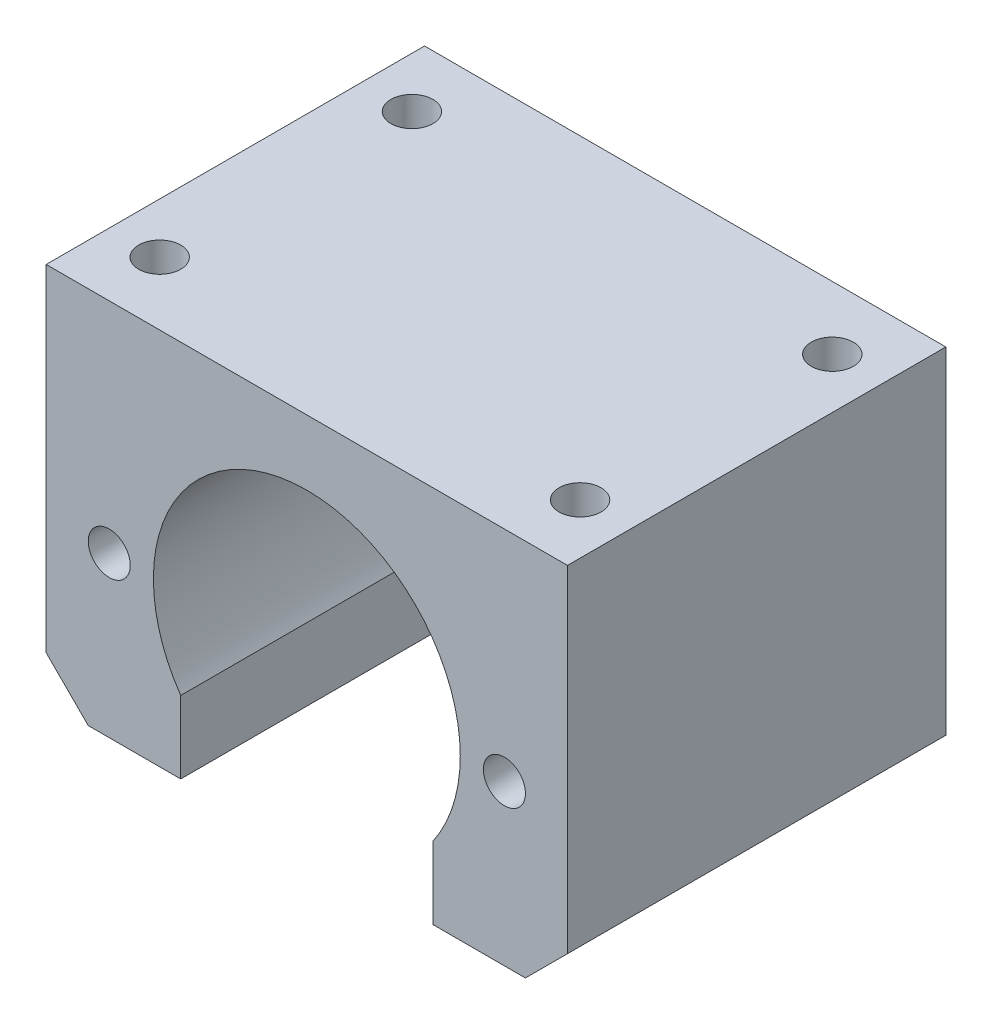
from build123d import *

# Parameters (mm, degrees)
SKETCH_1_W                  = 62
SKETCH_1_H                  = 45
EXTRUDE_1_DEPTH             = 22.5
CUT_EXTRUDE_1_DEPTH         = 45
CHAMFER_1_SIZE              = 5
HOLE_WIZARD_M6_1_D          = 5
HOLE_WIZARD_M6_1_DEPTH      = 15
HOLE_WIZARD_M6_1_TIP        = 1.502151548
HOLE_WIZARD_M6_2_AT_2_COUNT = 2
HOLE_WIZARD_M6_2_AT_2_PITCH = 47


with BuildPart() as part:
    # 草图1 → 凸台-拉伸1 (new, symmetric)
    with BuildSketch(Plane(origin=(0, 0, 0), x_dir=(1, 0, 0), z_dir=(0, 1, 0))):
        Rectangle(SKETCH_1_W, SKETCH_1_H)
    extrude(amount=EXTRUDE_1_DEPTH, both=True)

    # 草图2 → 切除-拉伸1 (cut)
    with BuildSketch(Plane(origin=(0, 0, -22.5), x_dir=(-1, 0, 0), z_dir=(0, 0, -1))):
        with BuildLine():
            Line((-15, -13.895311443), (-15, -22.5))
            Line((-15, -22.5), (15, -22.5))
            Line((15, -22.5), (15, -13.895311443))
            ThreePointArc((15, -13.895311443), (0, 14.75), (-15, -13.895311443))
        make_face()
    extrude(amount=-CUT_EXTRUDE_1_DEPTH, mode=Mode.SUBTRACT)

    # 倒角1
    chamfer_1_edges = [part.edges().sort_by_distance(p)[0] for p in [
        (-31, -22.5, 0),
        (31, -22.5, 0),
    ]]
    chamfer(chamfer_1_edges, length=CHAMFER_1_SIZE)

    # M6 螺纹孔1
    with Locations(Plane(origin=(0, 22.5, 0), x_dir=(1, 0, 0), z_dir=(0, 1, 0))):
        with Locations((-25, 15), (-25, -15), (25, -15), (25, 15)):
            Hole(HOLE_WIZARD_M6_1_D / 2, depth=HOLE_WIZARD_M6_1_DEPTH)
            with Locations((0, 0, -(HOLE_WIZARD_M6_1_DEPTH + HOLE_WIZARD_M6_1_TIP / 2))):  # 118° drill point
                Cone(0, HOLE_WIZARD_M6_1_D / 2, HOLE_WIZARD_M6_1_TIP, mode=Mode.SUBTRACT)

    # 草图6 → M6 螺纹孔2 (revolve, cut)
    with BuildSketch(Plane(origin=(23.5, -3.5, -22.5), x_dir=(0, 1, 0), z_dir=(1, 0, 0))):
        Polygon((0, 0), (0, 16.502151548), (2.5, 15), (2.5, 0), align=None)
    hole_wizard_m6_2 = revolve(axis=Axis((23.5, -3.5, -28.85), (0, 0, 1)), mode=Mode.SUBTRACT)

    # M6 螺纹孔2 at 2: M6 螺纹孔2 ×2
    with Locations(*[(-i * HOLE_WIZARD_M6_2_AT_2_PITCH, 0, 0) for i in range(1, HOLE_WIZARD_M6_2_AT_2_COUNT)]):
        add(hole_wizard_m6_2, mode=Mode.SUBTRACT)

    # 镜向1: M6 螺纹孔2 across plane
    add(hole_wizard_m6_2.mirror(Plane.XY), mode=Mode.SUBTRACT)

    # 镜向1 copy 1 sketch → 镜向1 copy 1 (revolve, cut)
    with BuildSketch(Plane(origin=(-23.5, -3.5, 22.5), x_dir=(0, 1, 0), z_dir=(1, 0, 0))):
        Polygon((0, 0), (0, -16.502151548), (2.5, -15), (2.5, 0), align=None)
    revolve(axis=Axis((-23.5, -3.5, 28.85), (0, 0, 1)), mode=Mode.SUBTRACT)


solid = part.part
